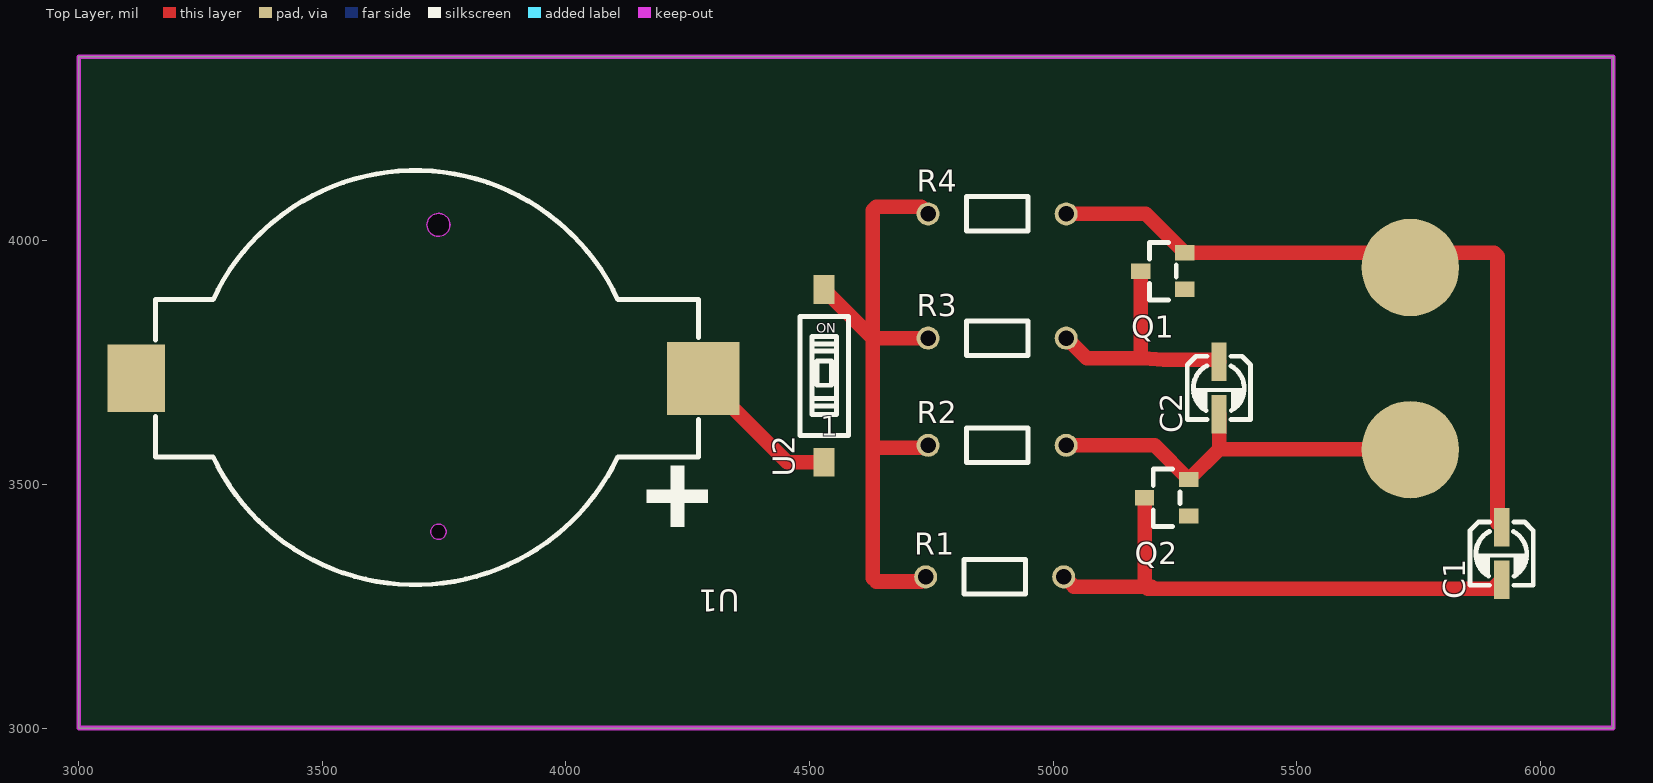
[diagram p0: Top Layer view]
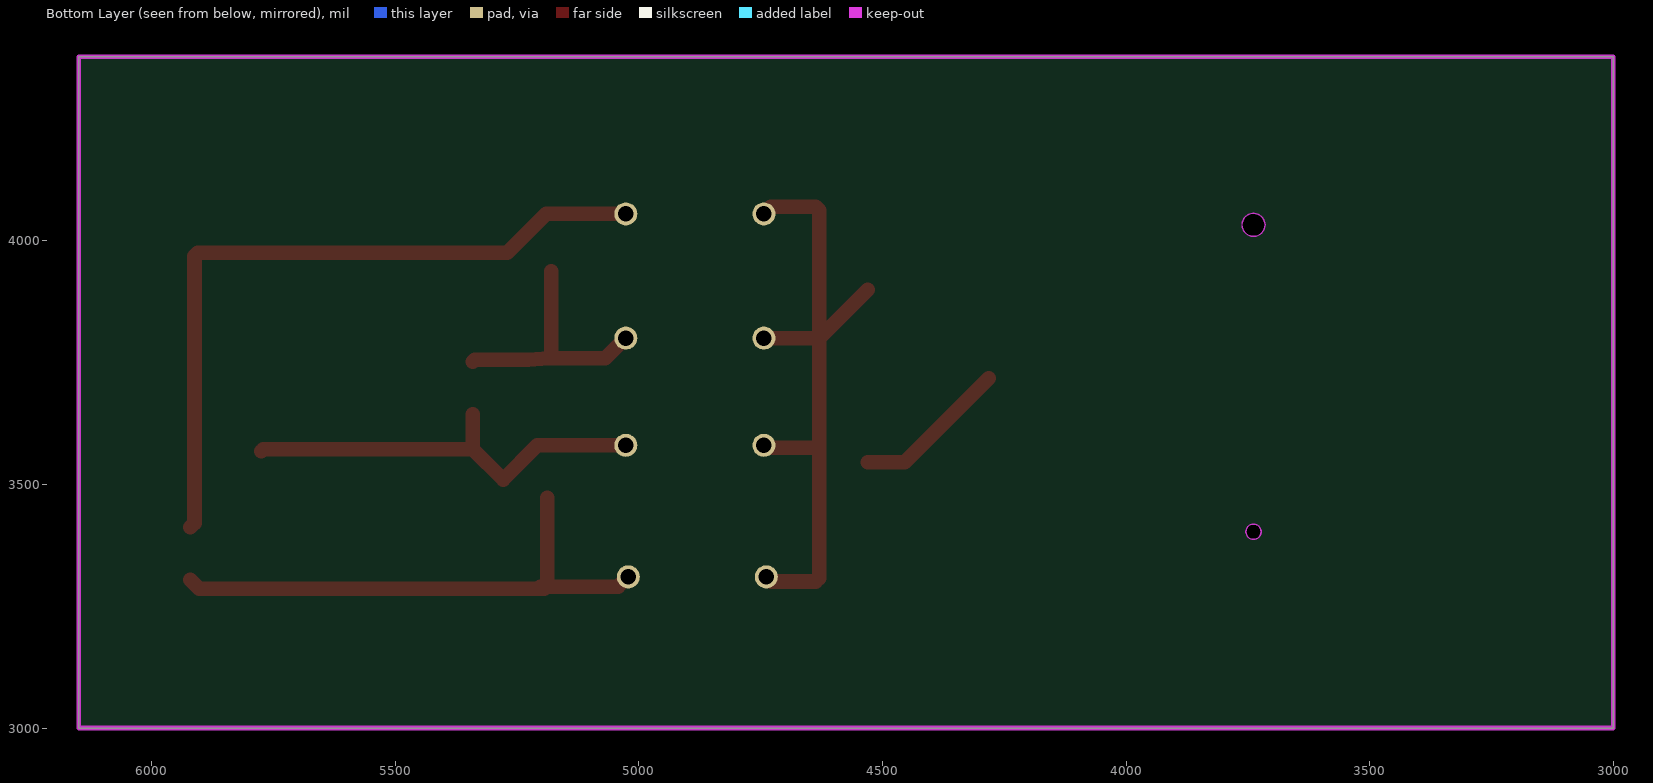
[diagram p1: Bottom Layer view, seen from below]
# Altium PCB MISC52073.pcbdoc
Units mil, origin at the board's own origin, x right, y up, seen from the top; angles counter-clockwise.
Board outline 3149.61 x 1377.95 mil, 2 copper layers (Top Layer, Bottom Layer), stack 62.206 mil thick; 10 components, 0 nets, 24 pads, 0 vias.

## Layer stack, top to bottom
Top Solder Mask Layer: solder mask 0.394, Dk 3.3
Top Layer: signal copper 1.379
Dielectric1: surface 59.449, FR4, Dk 4.5
Bottom Layer: signal copper 1.378
Bottom Solder Mask Layer: solder mask 0.394, Dk 3.3

## Board outline
3000,4377.95 3000,3000 6149.61,3000 6149.61,4377.95

## Design rules (kind name [scope] priority, off if disabled: settings)
BoardOutlineClearance copperThickness2oz_1 [All] p2 off: genericclearance=7.99 ignorepadtopadclearanceinfootprint=FALSE except(0: Arc-SplitContinuation Track-SplitContinuation SMDPad-SplitContinuation THPad-SplitContinuation Via-SplitContinuation Fill-SplitContinuation Region-SplitContinuation Poly-SplitContinuation Text-SplitContinuation Hole-SplitContinuation; 5.98: Arc-CutoutEdge SMDPad-CutoutEdge THPad-CutoutEdge Via-CutoutEdge Fill-CutoutEdge Region-CutoutEdge Text-CutoutEdge; 6.93: Hole-OutlineEdge Hole-CutoutEdge; 10: Poly-OutlineEdge Poly-CutoutEdge; 11.81: Arc-OutlineEdge Track-OutlineEdge SMDPad-OutlineEdge THPad-OutlineEdge Via-OutlineEdge Fill-OutlineEdge Region-OutlineEdge Text-OutlineEdge Track-CutoutEdge)
BoardOutlineClearance copperThickness1oz_1 [All] p4: genericclearance=4.02 ignorepadtopadclearanceinfootprint=FALSE except(0: Arc-SplitContinuation Track-SplitContinuation SMDPad-SplitContinuation THPad-SplitContinuation Via-SplitContinuation Fill-SplitContinuation Region-SplitContinuation Poly-SplitContinuation Text-SplitContinuation Hole-SplitContinuation; 6: SMDPad-CutoutEdge THPad-CutoutEdge Via-CutoutEdge Fill-CutoutEdge Region-CutoutEdge Text-CutoutEdge; 6.93: Hole-OutlineEdge Hole-CutoutEdge; 10: Poly-OutlineEdge Poly-CutoutEdge; 11.8: Arc-OutlineEdge Track-OutlineEdge SMDPad-OutlineEdge THPad-OutlineEdge Via-OutlineEdge Fill-OutlineEdge Region-OutlineEdge Text-OutlineEdge; 11.81: Arc-CutoutEdge Track-CutoutEdge)
Clearance copperThickness2oz [All] p1 off: gap=7.99 ignorepadtopadclearanceinfootprint=FALSE except(5.98: SMDPad-Track SMDPad-SMDPad THPad-Track SMDPad-THPad THPad-THPad Track-Via SMDPad-Via THPad-Via Via-Via Fill-Track Region-Track Fill-SMDPad Region-SMDPad Fill-THPad Region-THPad Fill-Via Region-Via Fill-Fill Fill-Region Region-Region Arc-Track Arc-SMDPad Arc-THPad Arc-Via Fill-Arc Region-Arc Arc-Arc Text-Track SMDPad-Text Text-THPad Text-Via Fill-Text Region-Text Arc-Text Text-Text; 6.93: Hole-Track Hole-SMDPad Hole-THPad Hole-Via Fill-Hole Region-Hole Hole-Arc Hole-Text; 10: Poly-Track Poly-SMDPad Poly-THPad Poly-Via Poly-Fill Poly-Region Poly-Poly Poly-Arc Poly-Text Poly-Hole)
Clearance copperThickness1oz [All] p3: gap=4.02 ignorepadtopadclearanceinfootprint=FALSE except(5.98: SMDPad-Track SMDPad-SMDPad THPad-Track SMDPad-THPad THPad-THPad Track-Via SMDPad-Via THPad-Via Via-Via Fill-Track Region-Track Fill-SMDPad Region-SMDPad Fill-THPad Region-THPad Fill-Via Region-Via Fill-Fill Fill-Region Region-Region; 6: Arc-Track Arc-SMDPad Arc-THPad Arc-Via Fill-Arc Region-Arc Arc-Arc Text-Track SMDPad-Text Text-THPad Text-Via Fill-Text Region-Text Arc-Text Text-Text; 6.93: Hole-Track Hole-SMDPad Hole-THPad Hole-Via Fill-Hole Region-Hole Hole-Arc Hole-Text; 10: Poly-Track Poly-SMDPad Poly-THPad Poly-Via Poly-Fill Poly-Region Poly-Poly Poly-Arc Poly-Text Poly-Hole)
DiffPairsRouting differentialPair [All] p1: maxlimit=6 minlimit=6 mostfreqgap=6 toplayer_minwidth=5 toplayer_prefwidth=10 toplayer_maxwidth=100 toplayer_mingap=6 toplayer_prefgap=6 toplayer_maxgap=6 bottomlayer_minwidth=5 bottomlayer_prefwidth=10 bottomlayer_maxwidth=100 bottomlayer_mingap=6 bottomlayer_prefgap=6 bottomlayer_maxgap=6 maxuncoupledlength=10
HoleToHoleClearance otherClearance [All] p1: gap=11.81 allowstackedmicrovias=TRUE
Length netLength [All] p1: minlimit=0 maxlimit=0
MatchedLengths netLengthTolerance [All] p1: tolerance=1000
PasteMaskExpansion pasteMaskExpansion [All] p1: expansion=0
PlaneConnect innerPlane [All] p1: planeconnectstyle=Relief reliefexpansion=20 reliefentries=4 reliefconductorwidth=10 reliefairgap=10
PolygonConnect copperRegion [All] p1: connectstyle=Relief reliefconductorwidth=10 reliefentries=4 polygonreliefangle="90 Angle" airgapwidth=10 via.connectstyle=Relief via.reliefconductorwidth=10 via.reliefentries=4 via.polygonreliefangle="90 Angle" via.airgapwidth=10
RoutingVias viaSize [All] p1: holewidth=12.01 width=24.02 viastyle="Through Hole" minholewidth=11.81 minwidth=19.68 maxholewidth=248.03 maxwidth=393.7
SolderMaskExpansion solderMaskExpansion [IsVia] p1: expansion=-1000 istentingtop=TRUE
SolderMaskExpansion solderMaskExpansion [All] p2: expansion=2 istentingtop=FALSE
Width copperThickness2oz_2 [All] p1 off: maxlimit=100 minlimit=8 preferedwidth=10
Width copperThickness1oz_2 [All] p2: maxlimit=100 minlimit=5 preferedwidth=10

## Components (designator, comment, footprint, x,y, rotation, side; value= is the part's Value field where it differs from the comment)
C1 "10uF" C_Ele_SMD_3x5.4mm 5920,3357.95 r90 top
C2 "10uF" C_Ele_SMD_3x5.4mm 5340,3697.95 r90 top
Q1 "" S8050_SOT-23 5225,3937.95 r0 top
Q2 "" S8050_SOT-23 5232.93,3472.87 r0 top
R1 "10kΩ" Res_1/8W 4880,3307.95 r0 top
R2 "10kΩ" Res_1/8W 4885,3577.95 r0 top
R3 "10kΩ" Res_1/8W 4885,3797.95 r0 top
R4 "10kΩ" Res_1/8W 4885,4052.95 r0 top
U1 "CR2032 battery holder" BAT-SMD_CR2032_C9900016310 3700,3717.95 r180 top
U2 "2.54-1P TPGT" SW-SMD_2P-L6.2-W2.5-LS9.4 4530,3722.95 r90 top

## Footprints (in the part's own frame and the unit in brackets; to place one, negate y for a bottom-side part, rotate by r counter-clockwise, add the part's x,y. Pads: shape width x height; smd on the part's side, far side on the other; paste and mask are expansions set on the pad)
BAT-SMD_CR2032_C9900016310 [mm]
  rect 3x3.5 smd paste+0 mask+0.05: 1(14.775,0)
  rect 3.8x3.8 smd paste+0 mask+0.05: 2(-14.775,0)
  Board Outline Layer circle w0.003: c-0.975,-8 r0.6
  Board Outline Layer circle w0.003: c-0.975,8 r0.4
  Board Outline Layer region: -1.575,-8 -1.516,-7.74 -1.349,-7.531 -1.108,-7.415 -0.841,-7.415 -0.601,-7.531 -0.434,-7.74 -0.375,-8 -0.375,-8 -0.434,-8.26 -0.601,-8.469 -0.841,-8.585 -1.108,-8.585 -1.349,-8.469 -1.516,-8.26 -1.575,-8
  Board Outline Layer region: -1.575,-8 -1.566,-7.896 -1.539,-7.795 -1.495,-7.7 -1.435,-7.614 -1.361,-7.54 -1.275,-7.48 -1.18,-7.436 -1.079,-7.409 -0.975,-7.4 -0.871,-7.409 -0.77,-7.436 -0.675,-7.48 -0.589,-7.54 -0.515,-7.614 -0.455,-7.7 -0.411,-7.795 -0.384,-7.896 -0.375,-8 -0.384,-8.104 -0.411,-8.205 -0.455,-8.3 -0.515,-8.386 -0.589,-8.46 -0.675,-8.52 -0.77,-8.564 -0.871,-8.591 -0.975,-8.6 -1.079,-8.591 -1.18,-8.564 -1.275,-8.52 -1.361,-8.46 -1.435,-8.386 -1.495,-8.3 -1.539,-8.205 -1.566,-8.104
  Board Outline Layer region: -1.375,8 -1.335,8.174 -1.224,8.313 -1.064,8.39 -0.886,8.39 -0.726,8.313 -0.615,8.174 -0.575,8 -0.575,8 -0.615,7.826 -0.726,7.687 -0.886,7.61 -1.064,7.61 -1.224,7.687 -1.335,7.826 -1.375,8
  Board Outline Layer region: -1.375,8 -1.365,8.089 -1.335,8.174 -1.288,8.249 -1.224,8.313 -1.149,8.36 -1.064,8.39 -0.975,8.4 -0.886,8.39 -0.801,8.36 -0.726,8.313 -0.662,8.249 -0.615,8.174 -0.585,8.089 -0.575,8 -0.585,7.911 -0.615,7.826 -0.662,7.751 -0.726,7.687 -0.801,7.64 -0.886,7.61 -0.975,7.6 -1.064,7.61 -1.149,7.64 -1.224,7.687 -1.288,7.751 -1.335,7.826 -1.365,7.911
  Multi-Layer board cut-out: -1.575,-8 -1.516,-7.74 -1.349,-7.531 -1.108,-7.415 -0.841,-7.415 -0.601,-7.531 -0.434,-7.74 -0.375,-8 -0.375,-8 -0.434,-8.26 -0.601,-8.469 -0.841,-8.585 -1.108,-8.585 -1.349,-8.469 -1.516,-8.26 -1.575,-8
  Multi-Layer board cut-out: -1.375,8 -1.335,8.174 -1.224,8.313 -1.064,8.39 -0.886,8.39 -0.726,8.313 -0.615,8.174 -0.575,8 -0.575,8 -0.615,7.826 -0.726,7.687 -0.886,7.61 -1.064,7.61 -1.224,7.687 -1.335,7.826 -1.375,8
  silkscreen extent -15.02,-10.83 13.78,10.76
C_Ele_SMD_3x5.4mm [mil]
  rect 78.7x31.5 smd paste+0 mask+2: 1(54.1,-0.55) 2(-53.7,-0.55)
  silkscreen extent -65,-65 65,65
Res_1/8W [mil]
  round 47.2 hole 31.5 paste+0 mask+2: 1(-141.7,2.48) 2(141.7,2.48)
  silkscreen extent -63,-33 63,38
S8050_SOT-23 [mm]
  rect 1x0.8 smd paste+0 mask+0.051: 1(1.15,-0.95) 2(1.15,0.95) 3(-1.15,0)
  silkscreen extent -0.7,-1.5 0.7,1.5
SW-SMD_2P-L6.2-W2.5-LS9.4 [mm]
  rect 1.5x1.1 smd: 1(-4.5,0) 2(4.5,0)
  silkscreen extent -3.1,-1.27 3.1,1.27

## Free pads (board coordinates)
  round 200 smd: 1(5733.1,3945.41) 2(5733.1,3571.51)

## Nets (pads, with @x,y where several pads share a name; then routed paths per layer and width w, separated by ;. In a path a pad name is that pad's centre, name@x,y a point inside that pad or via, vN(x,y) a via of type N, cw(c..) or ccw(c..) an arc to the next point about the centre after c; other vN are vias at no path point)
pads on no net: C1.1 C1.2 C2.1 C2.2 Q1.1 Q1.2 Q1.3 Q2.1 Q2.2 Q2.3 R1.1 R1.2 R2.1 R2.2 R3.1 R3.2 R4.1 R4.2 U1.1 U1.2 U2.1 U2.2
copper on no net: | length 5670.8
  Top Layer w30: 4281.69,3717.95 4453.86,3545.79 4530,3545.79 ; 4530,3900.12 4630,3800.12 ; 4738.3,3310.43 4728.75,3300.88 4637.07,3300.88 4630,3307.95 4630,3575.61 ; 4743.3,3580.43 4738.48,3575.61 4630,3575.61 ; 4743.3,3800.43 4742.99,3800.12 4630,3800.12 ; 4743.3,4055.43 4728.71,4070.02 4637.07,4070.02 4630,4062.95 4630,3800.12 ; 5018.72,3314.14 5042.9,3289.96 5190.64,3289.96 ; 5026.7,3580.43 5208.05,3580.43 5278.2,3510.27 5340.55,3572.62 ; 5026.7,4055.43 5190.2,4055.43 5270.28,3975.35 5905,3975.35 5912.07,3968.28 5912.07,3420.53 5920.55,3412.05 ; 5026.78,3800.85 5068.68,3758.95 5183.73,3758.95 ; 5179.72,3937.95 5179.72,3762.95 5183.73,3758.95 ; 5187.65,3472.87 5187.65,3292.95 5190.64,3289.96 ; 5202.45,3289.96 5190.64,3289.96 ; 5340.55,3644.25 5340.55,3572.62 ; 5340.55,3752.05 5336.72,3755.88 5226.62,3755.88 5183.73,3758.95 ; 5775,3567.95 5770.33,3572.62 5340.55,3572.62 ; 5920.55,3304.25 5902.18,3285.88 5194.72,3285.88 5190.64,3289.96 ; 4630,3575.61 4630,3800.12

## Keep-outs
Board Outline Layer:
  the board outline again, w10